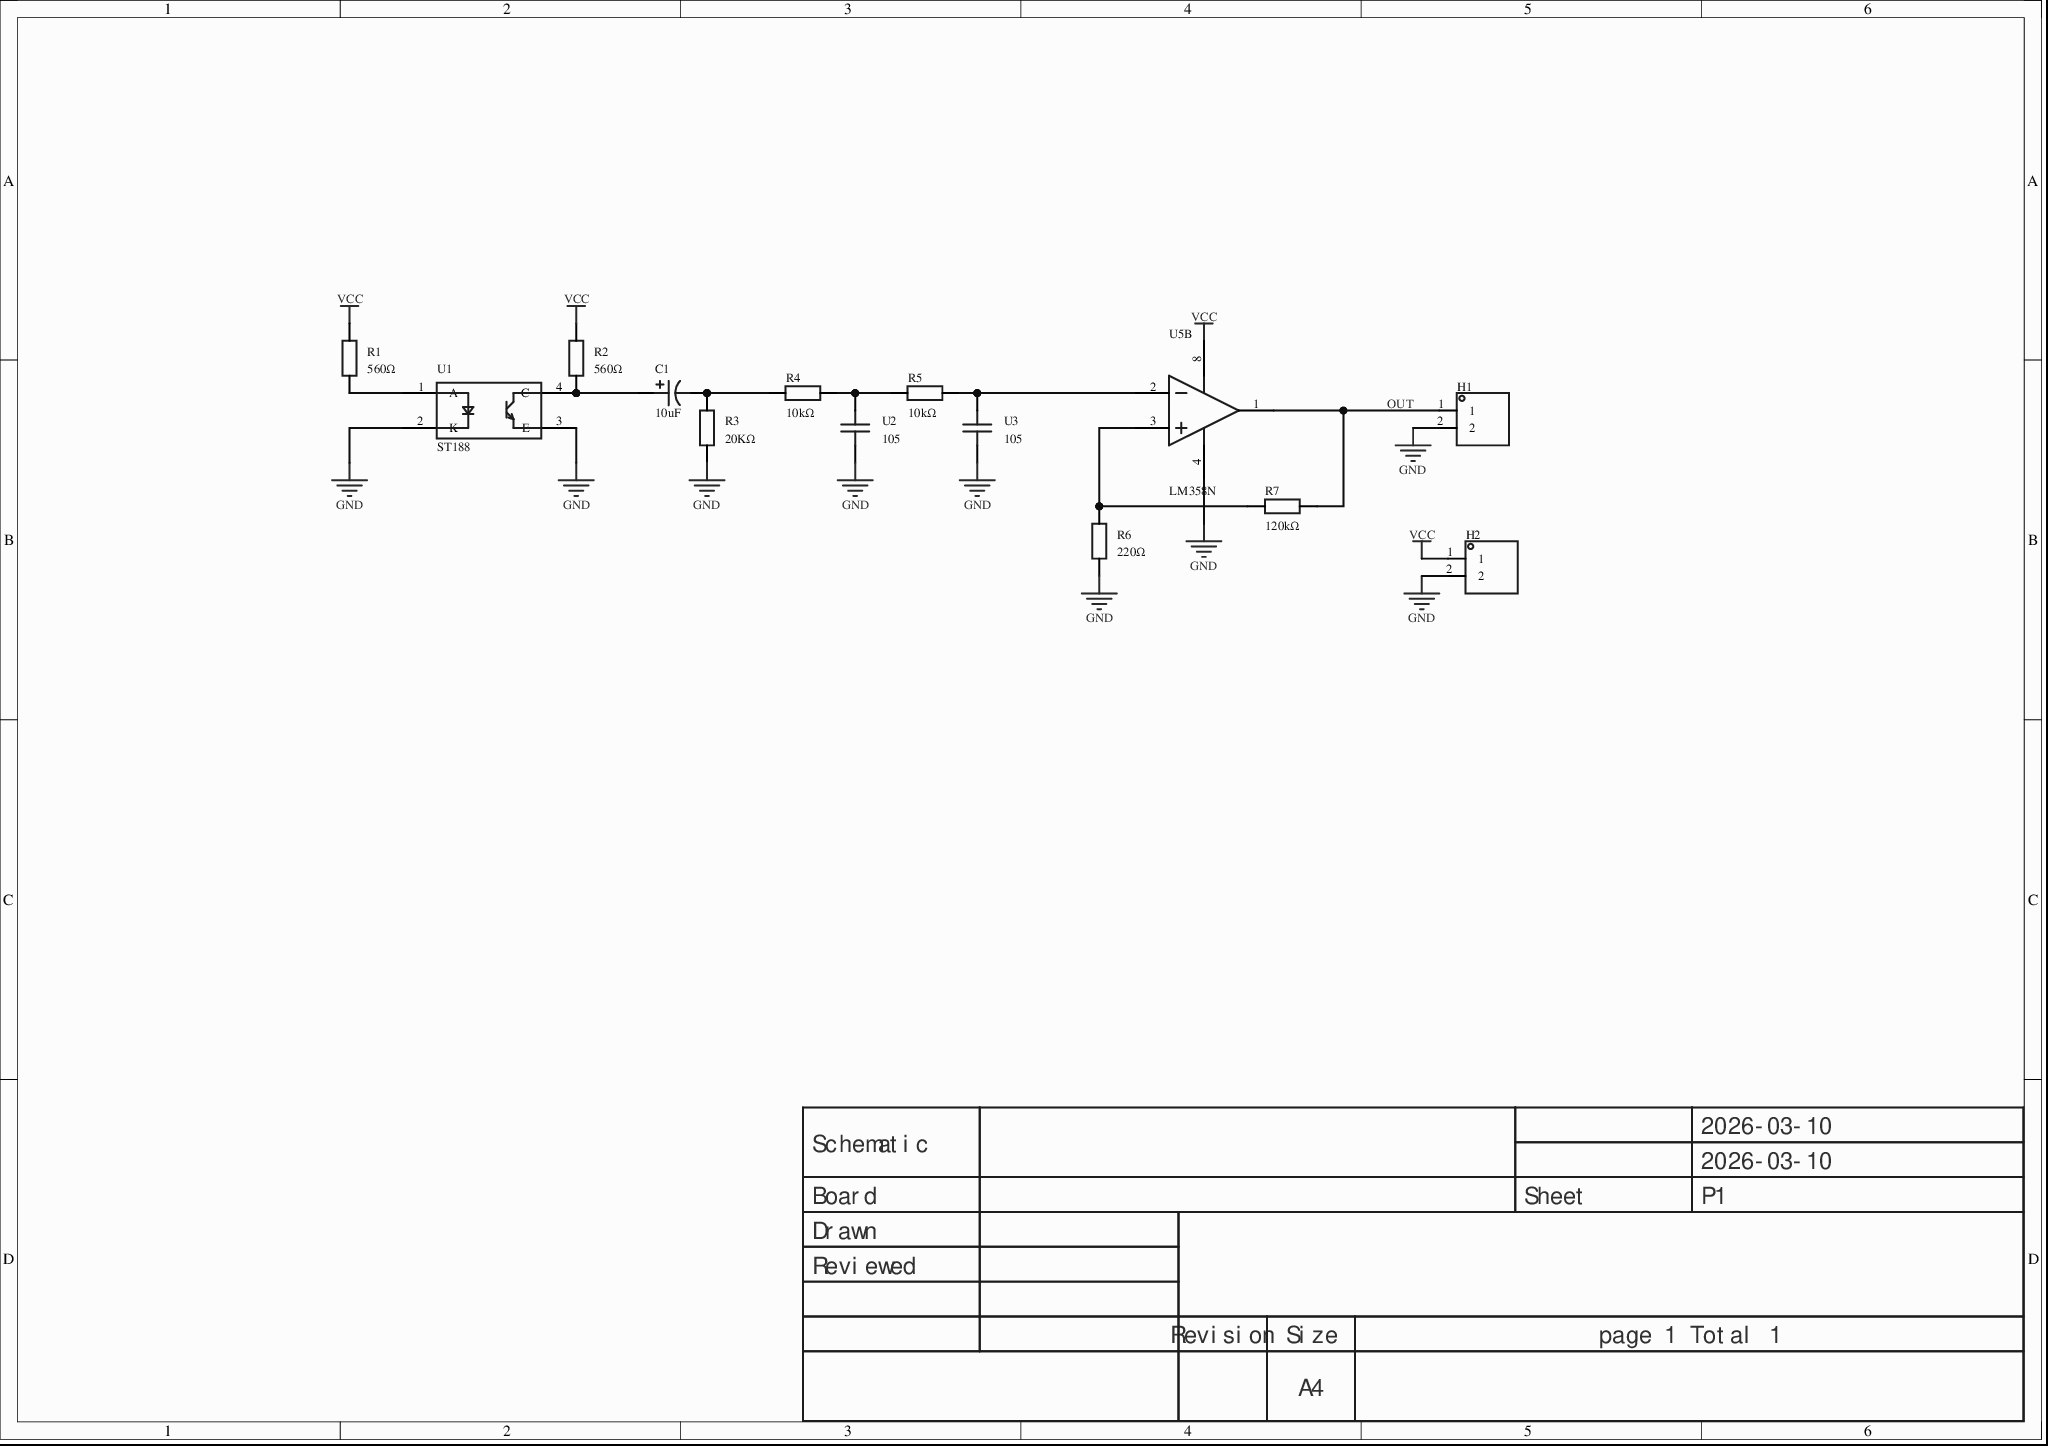
[diagram p0: MISC51900-3.schdoc]
# Altium project MISC51900-2.PrjPcb
1 sheet, 14 parts. Net scope: global (net labels, ports and power ports of the same name join across sheets).
Board file: MISC51900.pcbdoc

## Sheet MISC51900-3.schdoc
size 297 x 209 mm; Version: V1.0; @Project Name: MISC51900; @Update Date: 2026-03-10; @Create Date: 2026-03-10; @Board Name: MISC51900; @Create Time: 12:10:27; @Page Count: 1; @Page No: 1; @Schematic Name: MISC51900; @Update Time: 12:10:27; Size: A4

### Parts
C1  10uF  [CAP-TH_BD5.0-P2.00-D0.8-FD-10UF50VC110GL]
H1  (no value)  [HDR-TH_2P-P2.54-V-M-1]
H2  (no value)  [HDR-TH_2P-P2.54-V-M-1]
R1  560Ω  [Res_1/8W]
R2  560Ω  [Res_1/8W]
R3  20KΩ  [Res_1/8W]
R4  10kΩ  [Res_1/8W]
R5  10kΩ  [Res_1/8W]
R6  220Ω  [Res_1/8W]
R7  120kΩ  [Res_1/8W]
U1  ST188  [OPTO-TH_ST188]
U2  105  [CAP-TH_L5.0-W2.5-P5.00-D1.0]
U3  105  [CAP-TH_L5.0-W2.5-P5.00-D1.0]
U5  LM358N  [DIP-8_L9.2-W6.4-P2.54-LS7.6-BL]  (part B of 2)

### Nets
GND: H1.2 H2.2 R3.1 R6.1 U1.2(K) U1.3(E) U2.2 U3.2 U5.4(GND)
VCC: H2.1 R1.2 R2.2 U5.8(V+)
OUT: H1.1 R7.2 U5.1(OUTA)
NetC1_1: C1.1 R2.1 U1.4(C)
NetC1_2: C1.2 R3.2 R4.1
NetR1_1: R1.1 U1.1(A)
NetR4_2: R4.2 R5.1 U2.1
NetR5_2: R5.2 U3.1 U5.2(INA-)
NetR6_2: R6.2 R7.1 U5.3(INA+)

### Notes on the sheet
- 2026-03-10
- Schematic
- Board
- Sheet
- P1
- Drawn
- Reviewed
- Revision
- Size
- A4
- page 1 Total 1

### Library data of the parts
C1 = 10UF50VC110GL: Capacitance:10uF; Tolerance:±20%; Rated voltage:50V; Ripple current:120mA@100KHz; ESR:1.6Ω;; Manufacturer: Econd(米朗电子); AddInBom: yes; Tolerance: ±20%; Voltage Rating: 50V; Equivalent Series Resistance(ESR): 1.6Ω; Pin Spacing: 2mm; Lifetime: 5000hrs@105℃; Symbol: 10UF50VC110GL; Device: 10UF50VC110GL; LCSC Part Name: 10uF ±20% 50V; SupplierPart: C46867109; ManufacturerPart: 10UF50VC110GL; Supplier Footprint: 插件,D5xL11mm; JLCPCB Part Class: Extended Part; Datasheet: https://item.szlcsc.com/datasheet/10UF50VC110GL/49031974.html; Supplier: LCSC; ConvertToPcb: yes; FootprintName: CAP-TH_BD5.0-P2.00-D0.8-FD-10UF50VC110GL; Value: 10uF; Ripple Current: 120mA@100KHz; Diameter: 5mm; Height - Seated (Max): 11mm; Operating Temperature: -40℃~+105℃
H1 H2 = HDR-M_2.54_1x2P: Symbol: 210S-1*2P L=11.6MMGold-plated black; ConvertToPcb: yes; ModelId: 79b2e9f2d70a4d68a1b7098f27c6d4c50819f05c4eef4c71ace90d822a990e87; ModelName: HDR-M-2.54_1x2; ModelTransform: 200,100,0,0,0,0,0,0,-118.11; Device: HDR-M_2.54_1x2P; AddInBom: yes; SupplierPart: C124375; Supplier Footprint: 插件; FootprintName: HDR-TH_2P-P2.54-V-M-1
R1-R7 = Res_AXIAL-1/8W: Symbol: Resistor; ConvertToPcb: yes; ModelId: b2b5ae7ae4c642178fe0039925c86a3f0819f05c4eef4c71ace90d822a990e87; ModelName: RES-TH_BD1.8-L3.2-P7.20-D0.4; ModelTransform: 282.86,66.88,253.09,0,0,0,0,0,-191; Device: Res_AXIAL-1/8W; AddInBom: yes; Supplier Footprint: 轴向引线; FootprintName: Res_1/8W
  R1 R2: Value: 560Ω
  R3: Value: 20KΩ
  R4 R5: Value: 10kΩ
  R6: Value: 220Ω
  R7: Value: 120kΩ
U1 = ST188: AddInBom: yes; ModelId: 0c38d0078c35442caa51c7bd2cf255400819f05c4eef4c71ace90d822a990e87; ModelTransform: 370.078,216.535,0,0,0,0,0,0,-196.85; Symbol: ST188; Device: ST188; LCSC Part Name: ST188; SupplierPart: C9900004032; ManufacturerPart: ST188; Supplier Footprint: 插件; JLCPCB Part Class: Extended Part; Supplier: LCSC; ConvertToPcb: yes; FootprintName: OPTO-TH_ST188; ModelName: OPTO-TH_ST188
U2 U3 = 100nF: Symbol: 100NF_C9900015256; AddInBom: yes; ModelId: 08e3d7481fc7486bb1b263873f51e1e10819f05c4eef4c71ace90d822a990e87; ModelName: CAP-TH_BD5.0-W2.5-P5.08; ModelTransform: 224.652,98.425,0,0,0,0,-0.005,0,-137.795; Device: 100nF; Manufacturer Part: 105; LCSC Part Name: 100nF; SupplierPart: C9900015256; Supplier Footprint: CAP-TH_L5.0-W2.5-P5.00-D1.0; JLCPCB Part Class: Extended Part; Supplier: LCSC; ConvertToPcb: yes; FootprintName: CAP-TH_L5.0-W2.5-P5.00-D1.0
U5 = LM358N_C84858: Number of amplifiers: dual; Gain bandwidth product (GBP): 1MHz; Slew rate (SR): 0.6V/us;; Manufacturer: onsemi(安森美); Relevance: []; AddInBom: yes; ModelId: 0f67547f9f69422e93d8ef5b6ef310c70819f05c4eef4c71ace90d822a990e87; ModelTransform: 358.267,309.999,0,0,0,0,-0.004,0.002,-125.984; Symbol: LM358N_C84858; Device: LM358N_C84858; LCSC Part Name: LM358N 停产; SupplierPart: C84858; ManufacturerPart: LM358N; Supplier Footprint: DIP-8; JLCPCB Part Class: Extended Part; Datasheet: https://atta.szlcsc.com/upload/public/pdf/source/20180226/C84858_15196347430551369322.pdf; Supplier: LCSC; ConvertToPcb: yes; FootprintName: DIP-8_L9.2-W6.4-P2.54-LS7.6-BL; ModelName: DIP-8_L9.2-W6.4-P2.54-LS7.6-BL; Number of Circuits: Dual; Gain Bandwidth Product(GBP): 1MHz; Slew Rate(SR): 0.6V/us